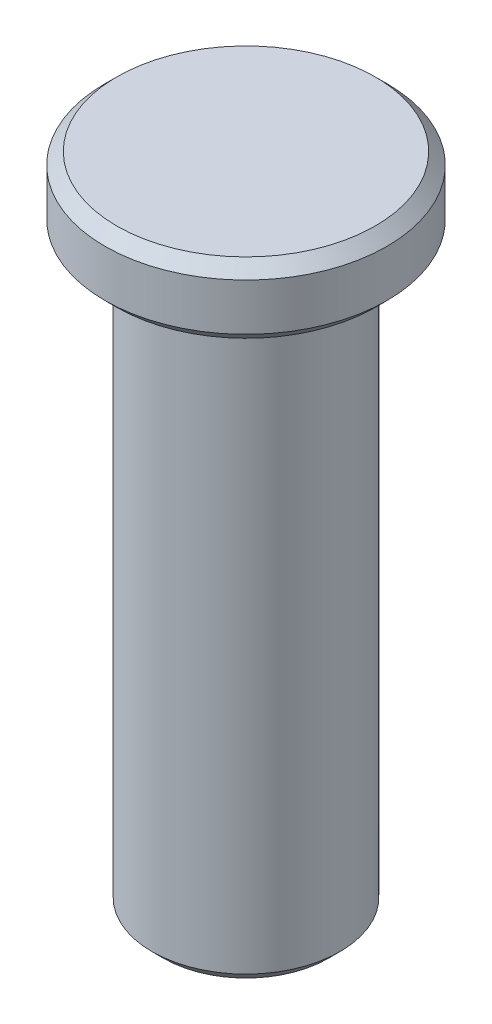
SolidWorks part; units mm, degrees
material "Q235-A"
ref_plane "Front Plane" through (0, 0, 0) normal (0, 0, 1) x (1, 0, 0)
ref_plane "Top Plane" through (0, 0, 0) normal (0, 1, 0) x (1, 0, 0)
ref_plane "Right Plane" through (0, 0, 0) normal (1, 0, 0) x (0, 0, -1)
sketch "Sketch2" plane through (0, 0, 0) normal (0, 1, 0) x (1, 0, 0)
  circle A0 centre (0, 0) radius 4
  dimension "D1" = 8
extrude "Boss-Extrude1" add sketch "Sketch2" along normal blind 25
sketch "Sketch3" plane through (0, 25, 0) normal (0, 1, 0) x (1, 0, 0)
  circle A0 centre (0, 0) radius 6
  dimension "D1" = 12
extrude "Boss-Extrude2" add sketch "Sketch3" along normal blind 3
chamfer "Chamfer1" distance 0.5 angle 45 3 edges at (0, 0, 4) (0, 25, 6) (0, 28, 6)
